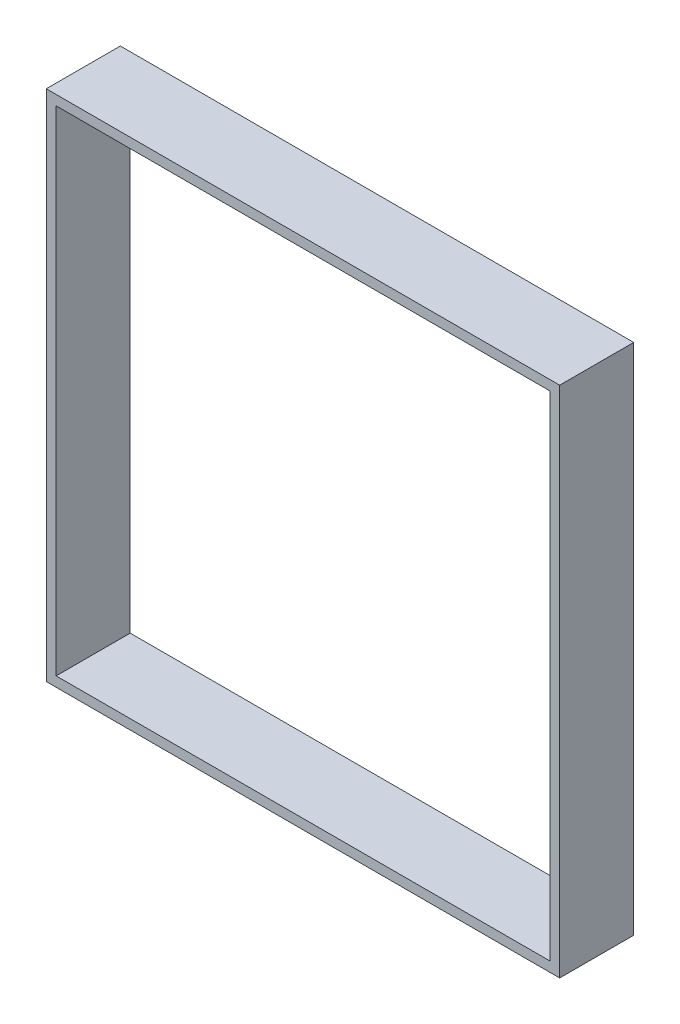
from build123d import *

# Parameters (mm, degrees)
SKETCH_1_W      = 208
SKETCH_1_H      = 208
SKETCH_1_W_2    = 200
SKETCH_1_H_2    = 200
EXTRUDE_1_DEPTH = 30


with BuildPart() as part:
    # 草图1 → 拉伸-薄壁1 (new body)
    with BuildSketch(Plane.XY):
        Rectangle(SKETCH_1_W, SKETCH_1_H)
        Rectangle(SKETCH_1_W_2, SKETCH_1_H_2, mode=Mode.SUBTRACT)
    extrude(amount=EXTRUDE_1_DEPTH)


solid = part.part
